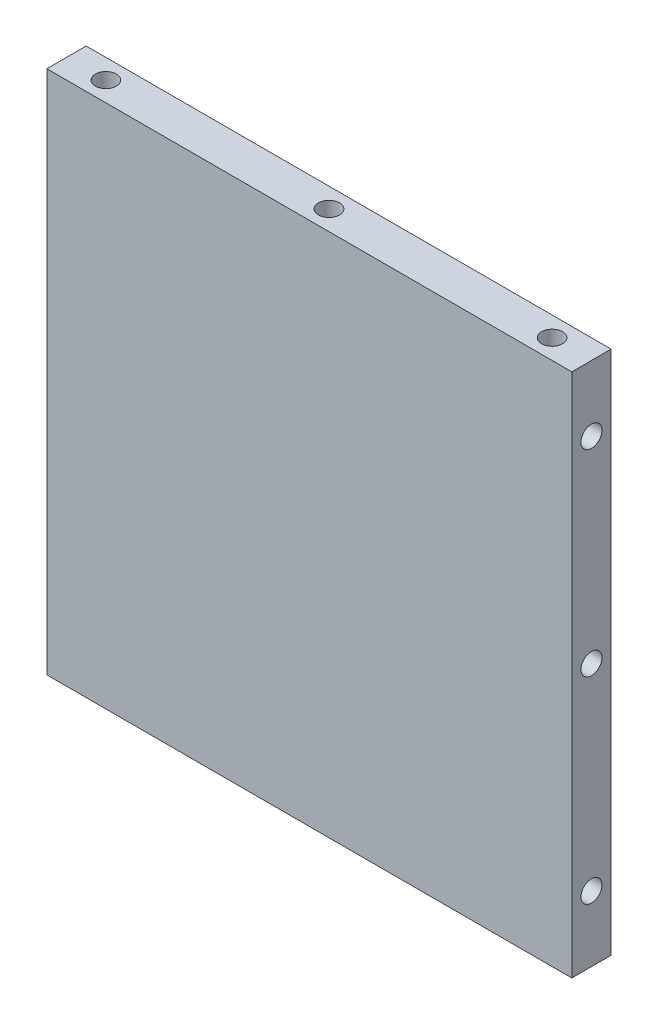
from build123d import *

# Parameters (mm, degrees)
SKETCH1_W               = 200
SKETCH1_H               = 200
BOSS_EXTRUDE1_DEPTH     = 15
SKETCH2_R               = 4
CUT_EXTRUDE1_DEPTH      = 25
LPATTERN1_COUNT         = 2
LPATTERN1_PITCH         = 75
MIRROR1_COPY_1_SKETCH_R = 4
MIRROR1_COPY_1_DEPTH    = 25
MIRROR2_COPY_1_SKETCH_R = 4
MIRROR2_COPY_1_DEPTH    = 25
MIRROR2_COPY_2_SKETCH_R = 4
MIRROR2_COPY_2_DEPTH    = 25
MIRROR2_COPY_3_SKETCH_R = 4
MIRROR2_COPY_3_DEPTH    = 25
SKETCH3_R               = 4
CUT_EXTRUDE2_DEPTH      = 25
LPATTERN2_COUNT         = 2
LPATTERN2_PITCH         = 85
MIRROR3_COPY_1_SKETCH_R = 4
MIRROR3_COPY_1_DEPTH    = 25
MIRROR4_COPY_1_SKETCH_R = 4
MIRROR4_COPY_1_DEPTH    = 25
MIRROR4_COPY_2_SKETCH_R = 4
MIRROR4_COPY_2_DEPTH    = 25
MIRROR4_COPY_3_SKETCH_R = 4
MIRROR4_COPY_3_DEPTH    = 25


with BuildPart() as part:
    # Sketch1 → Boss-Extrude1 (new body)
    with BuildSketch(Plane.XY):
        Rectangle(SKETCH1_W, SKETCH1_H)
    extrude(amount=BOSS_EXTRUDE1_DEPTH)

    # Sketch2 → Cut-Extrude1 (cut)
    with BuildSketch(Plane(origin=(100, 0, 0), x_dir=(0, 0, -1), z_dir=(1, 0, 0))):
        with Locations((-7.5, 0)):
            Circle(SKETCH2_R)
    cut_extrude1 = extrude(amount=-CUT_EXTRUDE1_DEPTH, mode=Mode.SUBTRACT)

    # LPattern1: Cut-Extrude1 ×2
    with Locations(*[(0, -i * LPATTERN1_PITCH, 0) for i in range(1, LPATTERN1_COUNT)]):
        add(cut_extrude1, mode=Mode.SUBTRACT)

    # Mirror1: Cut-Extrude1 across plane
    add(cut_extrude1.mirror(Plane.ZX), mode=Mode.SUBTRACT)

    # Mirror1 copy 1 sketch → Mirror1 copy 1 (cut)
    with BuildSketch(Plane(origin=(100, 75, 0), x_dir=(0, 0, -1), z_dir=(1, 0, 0))):
        with Locations((-7.5, 0)):
            Circle(MIRROR1_COPY_1_SKETCH_R)
    extrude(amount=-MIRROR1_COPY_1_DEPTH, mode=Mode.SUBTRACT)

    # Mirror2: Cut-Extrude1 across plane
    add(cut_extrude1.mirror(Plane(origin=(0, 0, 0), x_dir=(0, 0, 1), z_dir=(1, 0, 0))), mode=Mode.SUBTRACT)

    # Mirror2 copy 1 sketch → Mirror2 copy 1 (cut)
    with BuildSketch(Plane(origin=(-100, -75, 0), x_dir=(0, 0, -1), z_dir=(-1, 0, 0))):
        with Locations((-7.5, 0)):
            Circle(MIRROR2_COPY_1_SKETCH_R)
    extrude(amount=-MIRROR2_COPY_1_DEPTH, mode=Mode.SUBTRACT)

    # Mirror2 copy 2 sketch → Mirror2 copy 2 (cut)
    with BuildSketch(Plane(origin=(-100, 0, 0), x_dir=(0, 0, -1), z_dir=(-1, 0, 0))):
        with Locations((-7.5, 0)):
            Circle(MIRROR2_COPY_2_SKETCH_R)
    extrude(amount=-MIRROR2_COPY_2_DEPTH, mode=Mode.SUBTRACT)

    # Mirror2 copy 3 sketch → Mirror2 copy 3 (cut)
    with BuildSketch(Plane(origin=(-100, 75, 0), x_dir=(0, 0, -1), z_dir=(-1, 0, 0))):
        with Locations((-7.5, 0)):
            Circle(MIRROR2_COPY_3_SKETCH_R)
    extrude(amount=-MIRROR2_COPY_3_DEPTH, mode=Mode.SUBTRACT)

    # Sketch3 → Cut-Extrude2 (cut)
    with BuildSketch(Plane(origin=(0, 100, 0), x_dir=(1, 0, 0), z_dir=(0, 1, 0))):
        with Locations(Location((0, -7.5, 0), (0, 0, 180))):
            Circle(SKETCH3_R)
    cut_extrude2 = extrude(amount=-CUT_EXTRUDE2_DEPTH, mode=Mode.SUBTRACT)

    # LPattern2: Cut-Extrude2 ×2
    with Locations(*[(i * LPATTERN2_PITCH, 0, 0) for i in range(1, LPATTERN2_COUNT)]):
        add(cut_extrude2, mode=Mode.SUBTRACT)

    # Mirror3: Cut-Extrude2 across plane
    add(cut_extrude2.mirror(Plane(origin=(0, 0, 0), x_dir=(0, 0, 1), z_dir=(1, 0, 0))), mode=Mode.SUBTRACT)

    # Mirror3 copy 1 sketch → Mirror3 copy 1 (cut)
    with BuildSketch(Plane(origin=(-85, 100, 0), x_dir=(-1, 0, 0), z_dir=(0, 1, 0))):
        with Locations((0, 7.5)):
            Circle(MIRROR3_COPY_1_SKETCH_R)
    extrude(amount=-MIRROR3_COPY_1_DEPTH, mode=Mode.SUBTRACT)

    # Mirror4: Cut-Extrude2 across plane
    add(cut_extrude2.mirror(Plane.ZX), mode=Mode.SUBTRACT)

    # Mirror4 copy 1 sketch → Mirror4 copy 1 (cut)
    with BuildSketch(Plane(origin=(85, -100, 0), x_dir=(1, 0, 0), z_dir=(0, -1, 0))):
        with Locations((0, 7.5)):
            Circle(MIRROR4_COPY_1_SKETCH_R)
    extrude(amount=-MIRROR4_COPY_1_DEPTH, mode=Mode.SUBTRACT)

    # Mirror4 copy 2 sketch → Mirror4 copy 2 (cut)
    with BuildSketch(Plane(origin=(0, -100, 0), x_dir=(-1, 0, 0), z_dir=(0, -1, 0))):
        with Locations(Location((0, -7.5, 0), (0, 0, 180))):
            Circle(MIRROR4_COPY_2_SKETCH_R)
    extrude(amount=-MIRROR4_COPY_2_DEPTH, mode=Mode.SUBTRACT)

    # Mirror4 copy 3 sketch → Mirror4 copy 3 (cut)
    with BuildSketch(Plane(origin=(-85, -100, 0), x_dir=(-1, 0, 0), z_dir=(0, -1, 0))):
        with Locations(Location((0, -7.5, 0), (0, 0, 180))):
            Circle(MIRROR4_COPY_3_SKETCH_R)
    extrude(amount=-MIRROR4_COPY_3_DEPTH, mode=Mode.SUBTRACT)


solid = part.part
